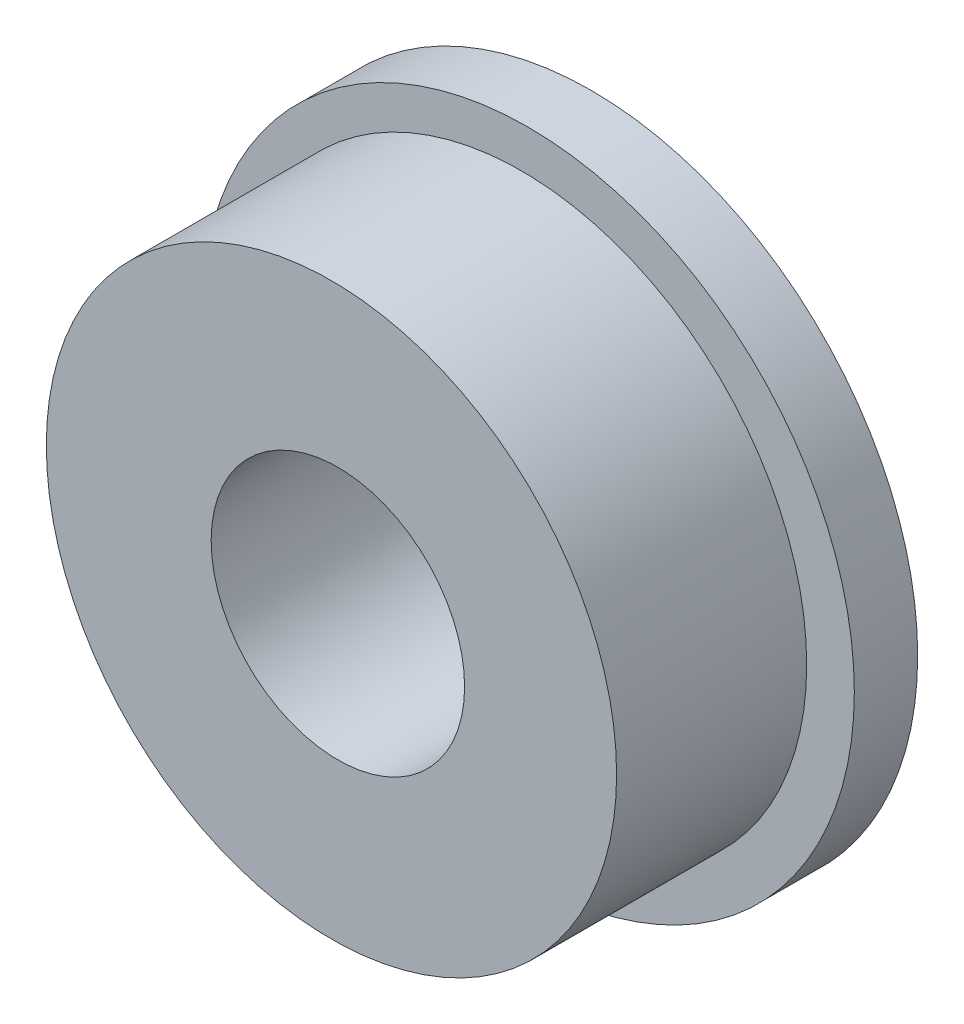
from build123d import *

# Parameters (mm, degrees)
SKETCH_1_R          = 5.15
SKETCH_1_R_2        = 2
EXTRUDE_1_DEPTH     = 4
CUT_EXTRUDE_START   = -3
SKETCH_2_R          = 5.15
SKETCH_2_R_2        = 4.5
CUT_EXTRUDE_1_DEPTH = 3


with BuildPart() as part:
    # 草图1 → 凸台-拉伸1 (new body)
    with BuildSketch(Plane.XY):
        Circle(SKETCH_1_R)
        Circle(SKETCH_1_R_2, mode=Mode.SUBTRACT)
    extrude(amount=EXTRUDE_1_DEPTH)

    # 草图2 → 切除-拉伸1 (cut)
    with BuildSketch(Plane.XY.offset(4).offset(CUT_EXTRUDE_START)):
        Circle(SKETCH_2_R)
        with Locations((-0.101257267, 0)):
            Circle(SKETCH_2_R_2, mode=Mode.SUBTRACT)
    extrude(amount=CUT_EXTRUDE_1_DEPTH, mode=Mode.SUBTRACT)


solid = part.part
